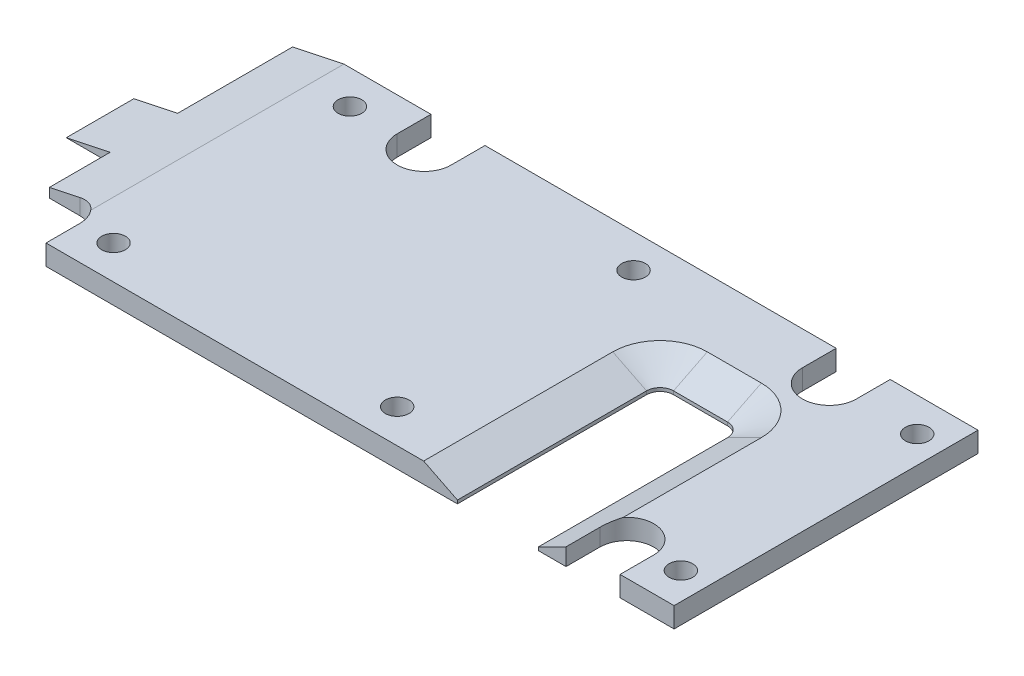
SolidWorks part; units mm, degrees
ref_plane "Front Plane" through (0, 0, 0) normal (0, 0, 1) x (1, 0, 0)
ref_plane "Top Plane" through (0, 0, 0) normal (0, 1, 0) x (1, 0, 0)
ref_plane "Right Plane" through (0, 0, 0) normal (1, 0, 0) x (0, 0, -1)
sketch "Sketch1" plane through (0, 0, 0) normal (0, 1, 0) x (1, 0, 0)
  line L1 (-52.25, 22.5) -> (52.25, 22.5)
  line L2 (-52.25, 22.5) -> (-52.25, -22.5)
  line L3 (-52.25, -22.5) -> (52.25, -22.5)
  line L4 (52.25, 22.5) -> (52.25, -22.5)
  line L5 (-52.25, 22.5) -> (52.25, -22.5) construction
  line L6 (-52.25, -22.5) -> (52.25, 22.5) construction
  point P0 (0, 0)
  dimension "D1" = 104.5
  dimension "D2" = 45
extrude "Boss-Extrude1" add sketch "Sketch1" along normal blind 3
sketch "Sketch2" plane through (0, 3, 0) normal (0, 1, 0) x (1, 0, 0)
  line L0 (23.17, 1.4905) -> (23.17, -49998.5095) construction
  line L1 (52.25, -22.5) -> (52.25, 22.5) construction
  line L2 (-52.25, -22.5) -> (52.25, -22.5) construction
  line L3 (17.17, 7.5) -> (29.17, 7.5)
  line L4 (17.17, 7.5) -> (17.17, -22.5)
  line L5 (17.17, -22.5) -> (29.17, -22.5)
  line L6 (29.17, 7.5) -> (29.17, -22.5)
  line L7 (17.17, 7.5) -> (29.17, -22.5) construction
  line L8 (17.17, -22.5) -> (29.17, 7.5) construction
  point P4 (23.17, -7.5)
  dimension "D1" = 29.08
  dimension "D2" = 12
  dimension "D3" = 30
extrude "Cut-Extrude1" cut sketch "Sketch2" against normal blind 34
sketch "Sketch3" plane through (0, 3, 0) normal (0, 1, 0) x (1, 0, 0)
  line L0 (29.17, -22.5) -> (52.25, -22.5) construction
  line L1 (52.25, 22.5) -> (49.25, 22.5)
  line L2 (52.25, 22.5) -> (52.25, -22.5)
  line L3 (52.25, -22.5) -> (49.25, -22.5)
  line L4 (49.25, 22.5) -> (49.25, -22.5)
  dimension "D1" = 3
extrude "Cut-Extrude2" cut sketch "Sketch3" against normal blind 10
sketch "Sketch4" plane through (0, 3, 0) normal (0, 1, 0) x (1, 0, 0)
  line L0 (-52.25, 0) -> (49947.75, 0) construction
  line L1 (-52.25, 22.5) -> (-52.25, -22.5) construction
  line L2 (49.25, 22.5) -> (49.25, -22.5) construction
  line L3 (49.25, 22.5) -> (-52.25, 22.5) construction
  line L4 (-34.75, 17.5) -> (49965.25, 17.5) construction
  line L5 (3.25, 17.5) -> (3.25, 50017.5) construction
  circle A0 centre (45.25, 17.5) radius 1.75
  circle A1 centre (45.25, -17.5) radius 1.75
  circle A2 centre (-38.75, 17.5) radius 1.75
  circle A3 centre (3.25, 17.5) radius 1.75
  circle A4 centre (-38.75, -17.5) radius 1.75
  circle A5 centre (3.25, -17.5) radius 1.75
  point P4 (-52.25, 0)
  dimension "D6" = 3.5
  dimension "D1" = 4
  dimension "D2" = 84
  dimension "D3" = 5
extrude "Cut-Extrude3" cut sketch "Sketch4" against normal blind 10
sketch "Sketch5" plane through (-52.25, 0, 0) normal (-1, 0, 0) x (0, 0, 1)
  line L0 (-22.5, 0) -> (22.5, 0) construction
  line L1 (-5.5, 0) -> (4.5, 0)
  line L2 (-5.5, 0) -> (-5.5, 3)
  line L3 (-5.5, 3) -> (4.5, 3)
  line L4 (4.5, 0) -> (4.5, 3)
  line L5 (-22.5, 3) -> (22.5, 3) construction
  line L6 (22.5, 3) -> (22.5, 0) construction
  line L7 (-0.5, 3) -> (-0.5, -49997) construction
  point P13 (-0.5, 3)
  point P14 (22.5, 1.5)
  dimension "D1" = 10
  dimension "D2" = 23
extrude "Boss-Extrude2" add sketch "Sketch5" along normal blind 6.5
sketch "Sketch6" plane through (0, 0, 22.5) normal (0, 0, 1) x (1, 0, 0)
  line L0 (-58.75, 0) -> (-44.6361, 3)
  line L1 (-52.25, 3) -> (17.17, 3) construction
  line L2 (-44.6361, 3) -> (-58.75, 3)
  line L3 (-58.75, 0) -> (-58.75, 3) construction
  line L4 (-58.75, 3) -> (-58.75, 0)
  dimension "D1" = 12
extrude "Cut-Extrude4" cut sketch "Sketch6" against normal through all
sketch "Sketch7" plane through (0, 3, 0) normal (0, 1, 0) x (1, 0, 0)
  line L0 (49.25, 22.5) -> (49.25, -22.5) construction
  line L1 (49.25, 22.5) -> (-44.6361, 22.5) construction
  line L8 (29.17, -22.5) -> (49.25, -22.5) construction
  circle A0 centre (-27.75, 17.5) radius 4
  circle A1 centre (-47.75, -17.5) radius 4
  circle A2 centre (32.25, 17.5) radius 4
  circle A3 centre (37.25, -17.5) radius 4
  point P14 (-27.75, 21.5)
  dimension "D5" = 8
  dimension "D6" = 5
  dimension "D7" = 5
  dimension "D1" = 60
  dimension "D2" = 17
  dimension "D3" = 12
  dimension "D4" = 85
extrude "Cut-Extrude5" cut sketch "Sketch7" against normal blind 10
sketch "Sketch8" plane through (0, 3, 0) normal (0, 1, 0) x (1, 0, 0)
  line L0 (-23.75, 17.5) -> (-23.75, 26.1682)
  line L1 (-31.75, 17.5) -> (-31.75, 26.1682)
  line L2 (-31.75, 26.1682) -> (-23.75, 26.1682)
  line L3 (36.25, 17.5) -> (36.25, 26.1682)
  line L4 (28.25, 17.5) -> (28.25, 26.1682)
  line L5 (28.25, 26.1682) -> (36.25, 26.1682)
  line L6 (41.25, -17.5) -> (41.25, -22.5)
  line L7 (29.17, -22.5) -> (49.25, -22.5) construction
  line L8 (33.25, -17.5) -> (33.25, -22.5)
  line L10 (-43.75, -17.5) -> (-43.75, -22.5)
  line L11 (-44.6361, -22.5) -> (17.17, -22.5) construction
  line L12 (-47.75, -13.5) -> (-52.25, -13.5)
  line L13 (-52.25, -22.5) -> (-52.25, -4.5) construction
  line L14 (-43.75, -22.5) -> (-52.25, -22.5)
  line L15 (-52.25, -22.5) -> (-52.25, -13.5)
  line L16 (33.25, -22.5) -> (41.25, -22.5)
  line L17 (36.25, 17.5) -> (28.25, 17.5)
  line L18 (-23.75, 17.5) -> (-31.75, 17.5)
  circle A0 centre (-27.75, 17.5) radius 4 construction
  circle A1 centre (32.25, 17.5) radius 4 construction
  circle A2 centre (37.25, -17.5) radius 4 construction
  arc A4 (-44.6361, -20.0107) -> (-44.6361, -14.9893) centre (-47.75, -17.5) ccw construction
  arc A5 (-44.6361, -14.9893) -> (-44.6361, -20.0107) centre (-47.75, -17.5) ccw construction
  arc A6 (-43.75, -17.5) -> (-47.75, -13.5) centre (-47.75, -17.5) ccw
  arc A7 (41.25, -17.5) -> (33.25, -17.5) centre (37.25, -17.5) ccw
extrude "Cut-Extrude6" cut sketch "Sketch8" against normal blind 10
fillet "Fillet1" radius 2 2 edges at (29.17, 1.5, -7.5) (17.17, 1.5, -7.5)
chamfer "Chamfer2" distance 5 distance2 2.5 5 edges at (29.17, 3, 8.5) (28.5842, 3, -6.9142) (23.17, 3, -7.5) (17.7558, 3, -6.9142) (17.17, 3, 8.5)
